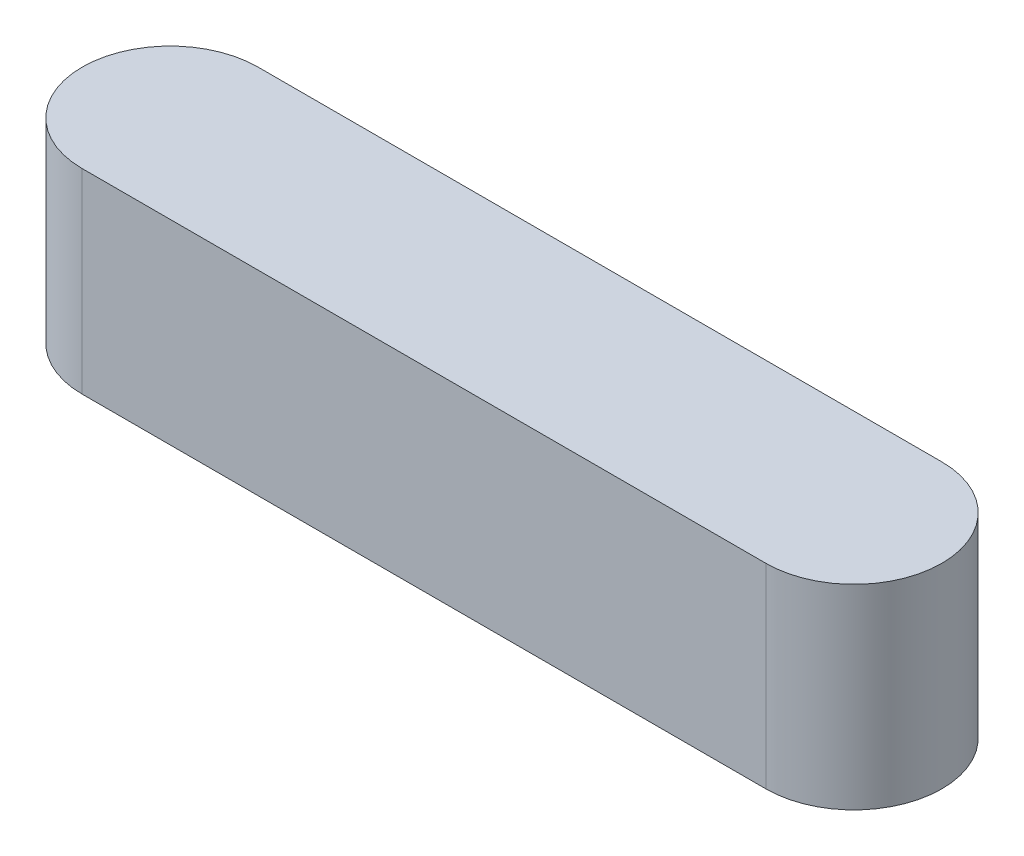
SolidWorks part; units mm, degrees
ref_plane "Front" through (0, 0, 0) normal (0, 0, 1) x (1, 0, 0)
ref_plane "Top" through (0, 0, 0) normal (0, 1, 0) x (1, 0, 0)
ref_plane "Right" through (0, 0, 0) normal (1, 0, 0) x (0, 0, -1)
sketch "Sketch1" plane through (0, 0, 0) normal (0, 1, 0) x (1, 0, 0)
  line L0 (0, 0) -> (35, 0) construction
  line L1 (0, 4.5) -> (35, 4.5)
  line L2 (0, -4.5) -> (35, -4.5)
  arc A0 (0, 4.5) -> (0, -4.5) centre (0, 0) ccw
  arc A1 (35, -4.5) -> (35, 4.5) centre (35, 0) ccw
  point P3 (17.5, 0)
  dimension "D2" = 4.5
  dimension "D1" = 35
extrude "Boss-Extrude1" add sketch "Sketch1" along normal blind 10
scale "Scale 1" bodies to scale 101 scale about centroid uniform scaling yes scale factor 1.875
